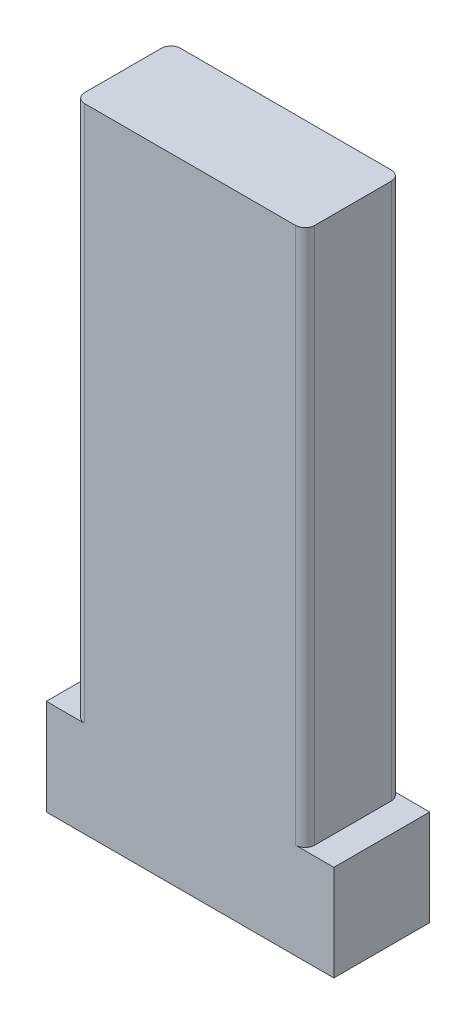
from build123d import *

# Parameters (mm, degrees)
SKETCH1_W           = 15
SKETCH1_H           = 5
BOSS_EXTRUDE1_DEPTH = 2.5
SKETCH3_W           = 12
SKETCH3_H           = 5
BOSS_EXTRUDE2_DEPTH = 28
FILLET1_R           = 0.5


with BuildPart() as part:
    # Sketch1 → Boss-Extrude1 (new, symmetric)
    with BuildSketch(Plane.XY):
        with Locations((0, -52.27)):
            Rectangle(SKETCH1_W, SKETCH1_H)
    extrude(amount=BOSS_EXTRUDE1_DEPTH, both=True)

    # Sketch3 → Boss-Extrude2 (add)
    with BuildSketch(Plane(origin=(0, -49.77, 0), x_dir=(1, 0, 0), z_dir=(0, 1, 0))):
        Rectangle(SKETCH3_W, SKETCH3_H)
    extrude(amount=BOSS_EXTRUDE2_DEPTH)

    # Fillet1
    fillet1_edges = [part.edges().sort_by_distance(p)[0] for p in [
        (-6, -35.77, -2.5),
        (-6, -35.77, 2.5),
        (6, -35.77, 2.5),
        (6, -35.77, -2.5),
    ]]
    fillet(fillet1_edges, radius=FILLET1_R)


solid = part.part
